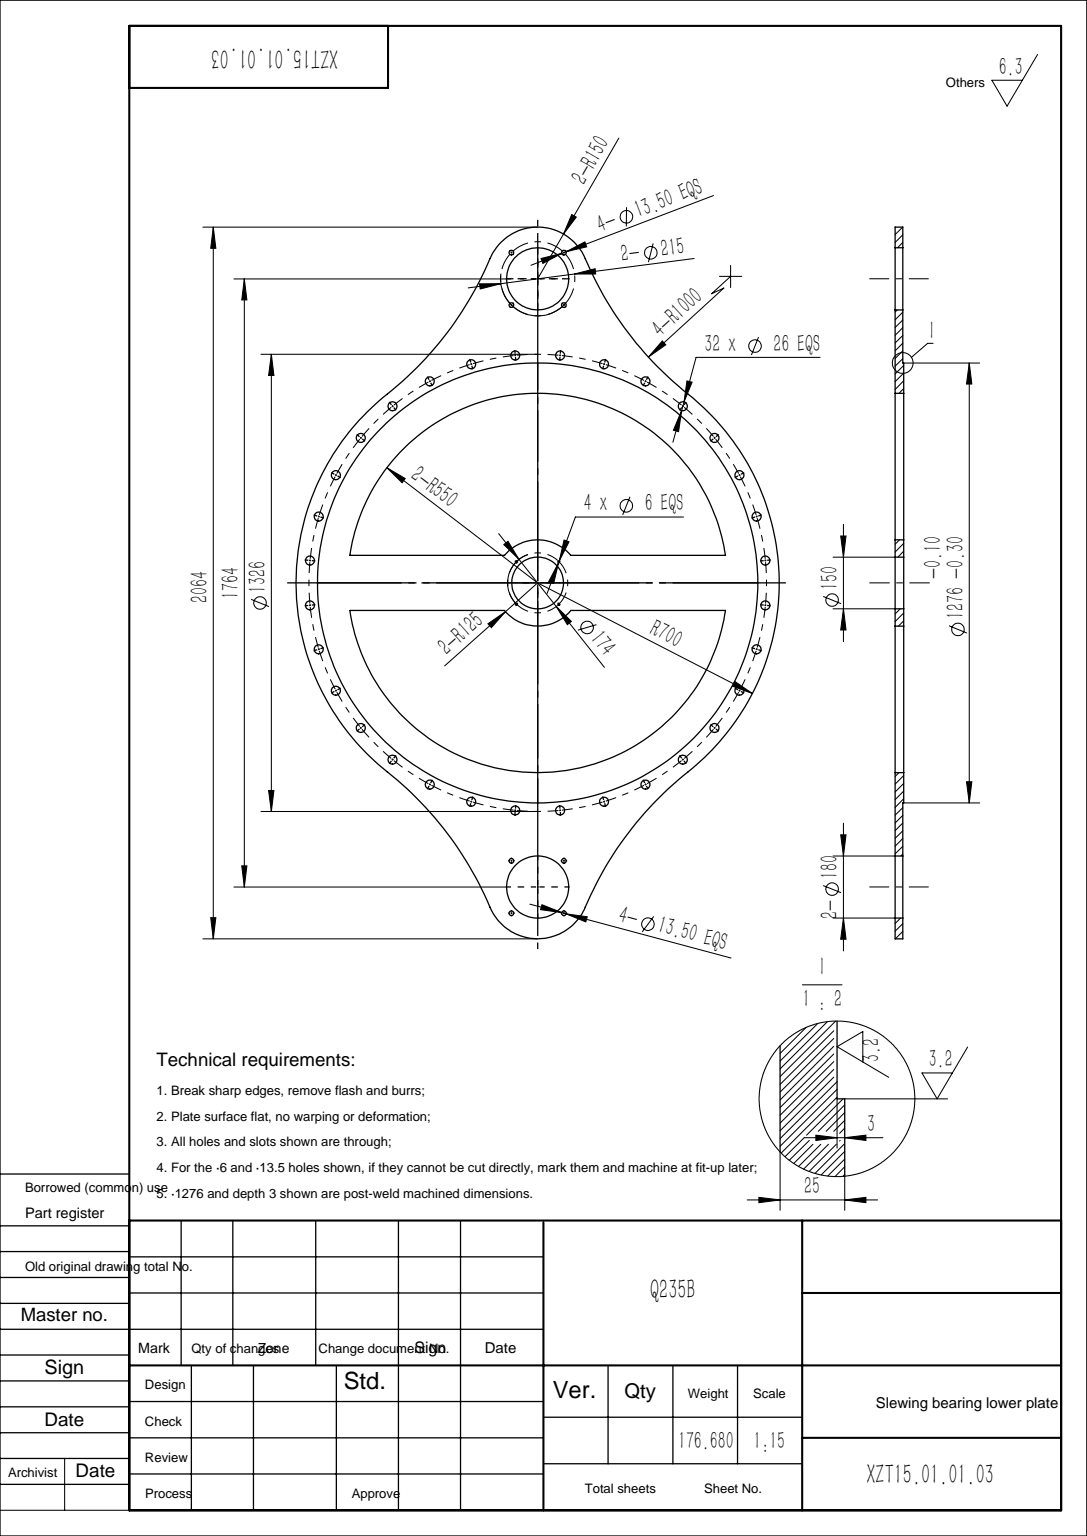
SolidWorks part; units mm, degrees
material "Q235B"
ref_plane "Front Plane" through (0, 0, 0) normal (0, 0, 1) x (1, 0, 0)
ref_plane "Top Plane" through (0, 0, 0) normal (0, 1, 0) x (1, 0, 0)
ref_plane "Right Plane" through (0, 0, 0) normal (1, 0, 0) x (0, 0, -1)
sketch "Sketch1" plane through (0, 0, 0) normal (0, 1, 0) x (1, 0, 0)
  line L0 (0, 882) -> (0, 0) construction
  line L1 (600, -80) -> (-600, -80)
  line L2 (600, -80) -> (600, 80)
  line L3 (600, 80) -> (-600, 80)
  line L4 (-600, -80) -> (-600, 80)
  line L5 (600, -80) -> (-600, 80) construction
  line L6 (600, 80) -> (-600, -80) construction
  line L7 (0, 0) -> (-1185.6839, 0) construction
  circle A0 centre (0, 0) radius 700
  circle A1 centre (0, 0) radius 550
  circle A2 centre (0, 0) radius 125
  circle A3 centre (0, 882) radius 150
  arc A4 (-436.1887, 547.4846) -> (-138.1716, 940.3833) centre (-1059.3155, 1329.6054) ccw
  arc A5 (436.1887, 547.4846) -> (138.1716, 940.3833) centre (1059.3155, 1329.6054) cw
  circle A6 centre (0, 882) radius 90
  circle A7 centre (0, -882) radius 90
  arc A8 (436.1887, -547.4846) -> (138.1716, -940.3833) centre (1059.3155, -1329.6054) ccw
  arc A9 (-436.1887, -547.4846) -> (-138.1716, -940.3833) centre (-1059.3155, -1329.6054) cw
  circle A10 centre (0, -882) radius 150
  circle A11 centre (0, 0) radius 75
  dimension "D1" = 1400
  dimension "D2" = 1100
  dimension "D5" = 250
  dimension "D6" = 300
  dimension "D7" = 1000
  dimension "D9" = 180
  dimension "D10" = 150
  dimension "D3" = 160
  dimension "D4" = 1200
  dimension "D8" = 1764
extrude "Boss-Extrude1" add sketch "Sketch1" along normal blind 25 contours A0 A5 A3 A4 | A3 A6 | A0 A1 L3 L2 L1 L4 | A1 L3 L4 L1 | A2 L3 A1 L1 | A2 L1 A1 L3 | A1 L1 L2 L3 | A9 A10 A8 A0 | A10 A7 | A11 L1 A2 | A11 L3 A2 L1 | A11 L3 A2
sketch "Sketch2" plane through (0, 25, 0) normal (0, 1, 0) x (1, 0, 0)
  circle A0 centre (0, 0) radius 638
  dimension "D1" = 1276
extrude "Cut-Extrude1" cut sketch "Sketch2" against normal blind 3 flip side to cut
hole_wizard "Ø24.5 (24.5) Diameter Hole1" positions "Sketch3" profile "Sketch4" hole size "Ø24.5" standard "GB" end condition up to next
sketch "Sketch3" plane through (0, 22, 0) normal (0, 1, 0) x (1, 0, 0)
  line L0 (0, 0) -> (659.8075, 64.9854) construction
  line L2 (0, 0) -> (659.8075, 64.9854) construction
  line L3 (0, 0) -> (663, 0) construction
  circle A0 centre (0, 0) radius 663 construction
  point P0 (659.8075, 64.9854)
  point P15 (659.8075, -64.9854)
  point P16 (634.4514, -192.4587)
  point P17 (584.7138, -312.536)
  point P18 (512.5059, -420.6027)
  point P19 (420.6027, -512.5059)
  point P20 (312.536, -584.7138)
  point P21 (192.4587, -634.4514)
  point P22 (64.9854, -659.8075)
  point P23 (-64.9854, -659.8075)
  point P24 (-192.4587, -634.4514)
  point P25 (-312.536, -584.7138)
  point P26 (-420.6027, -512.5059)
  point P27 (-512.5059, -420.6027)
  point P28 (-584.7138, -312.536)
  point P29 (-634.4514, -192.4587)
  point P30 (-659.8075, -64.9854)
  point P31 (-659.8075, 64.9854)
  point P32 (-634.4514, 192.4587)
  point P33 (-584.7138, 312.536)
  point P34 (-512.5059, 420.6027)
  point P35 (-420.6027, 512.5059)
  point P36 (-312.536, 584.7138)
  point P37 (-192.4587, 634.4514)
  point P38 (-64.9854, 659.8075)
  point P39 (64.9854, 659.8075)
  point P40 (192.4587, 634.4514)
  point P41 (312.536, 584.7138)
  point P42 (420.6027, 512.5059)
  point P43 (512.5059, 420.6027)
  point P44 (584.7138, 312.536)
  point P45 (634.4514, 192.4587)
  dimension "D1" = 1326
  dimension "D4" = 663
  dimension "D3" = 32
sketch "Sketch4" plane through (659.8075, 22, -64.9854) normal (1, 0, 0) x (0, 0, 1)
  line L0 (0, 0) -> (0, 22)
  line L1 (0, 22) -> (13, 22)
  line L2 (13, 22) -> (13, 0)
  line L5 (13, 0) -> (0, 0)
  line L11 (0, -6.35) -> (0, 107.95) construction
  dimension "通孔孔直径" = 26
  dimension "通孔孔深度" = 22
hole_wizard "Ø6.0 (6) Diameter Hole1" positions "Sketch5" profile "Sketch6" hole size "Ø6.0" standard "GB" end condition up to next
sketch "Sketch5" plane through (0, 25, 0) normal (0, 1, 0) x (1, 0, 0)
  line L0 (0, 0) -> (-61.5183, 61.5183) construction
  line L2 (0, 0) -> (-61.5183, 61.5183) construction
  circle A0 centre (0, 0) radius 87
  point P0 (-61.5183, 61.5183)
  point P17 (61.5183, 61.5183)
  point P18 (61.5183, -61.5183)
  point P19 (-61.5183, -61.5183)
  dimension "D1" = 174
  dimension "D2" = 45
  dimension "D4" = 87
  dimension "D3" = 4
sketch "Sketch6" plane through (-61.5183, 25, -61.5183) normal (1, 0, 0) x (0, 0, 1)
  line L0 (0, 0) -> (0, 25)
  line L1 (0, 25) -> (3, 25)
  line L2 (3, 25) -> (3, 0)
  line L5 (3, 0) -> (0, 0)
  line L11 (0, -6.35) -> (0, 107.95) construction
  dimension "通孔孔直径" = 6
  dimension "通孔孔深度" = 25
hole_wizard "Ø13.5 (13.5) Diameter Hole1" positions "Sketch7" profile "Sketch8" hole size "Ø13.5" standard "GB" end condition up to next
sketch "Sketch7" plane through (0, 22, 0) normal (0, 1, 0) x (1, 0, 0)
  line L0 (0, 882) -> (-76.014, 958.014) construction
  line L2 (0, 882) -> (-76.014, 958.014) construction
  circle A0 centre (0, 882) radius 107.5 construction
  point P0 (-76.014, 958.014)
  point P17 (76.014, 958.014)
  point P18 (76.014, 805.986)
  point P19 (-76.014, 805.986)
  dimension "D1" = 215
  dimension "D2" = 45
  dimension "D4" = 107.5
  dimension "D3" = 4
sketch "Sketch8" plane through (-76.014, 22, -958.014) normal (1, 0, 0) x (0, 0, 1)
  line L0 (0, 0) -> (0, 22.001)
  line L1 (0, 22.001) -> (6.75, 22.001)
  line L2 (6.75, 22.001) -> (6.75, 0)
  line L5 (6.75, 0) -> (0, 0)
  line L11 (0, -6.35) -> (0, 107.95) construction
  dimension "通孔孔直径" = 13.5
  dimension "通孔孔深度" = 22.001
mirror "Mirror1" about plane through (0, 0, 0) normal (0, 0, 1) of "Ø13.5 (13.5) Diameter Hole1"
